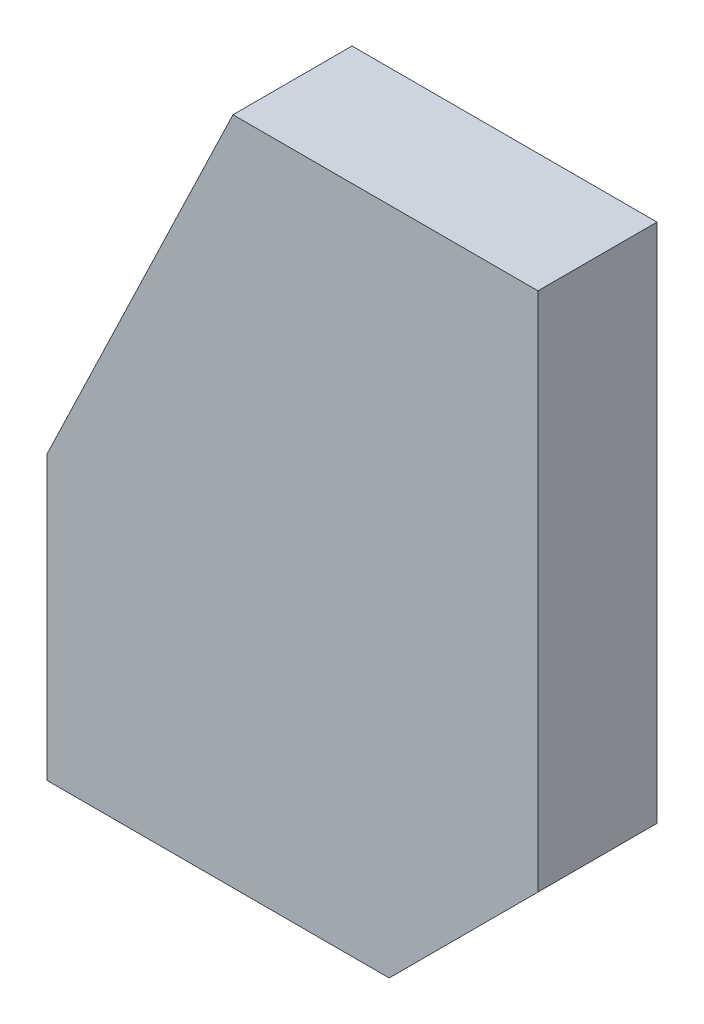
from build123d import *

# Parameters (mm, degrees)
EXTRUDE_1_DEPTH = 8
CHAMFER_1_SIZE  = 20


with BuildPart() as part:
    # 草图2 → 凸台-拉伸1 (new, symmetric)
    with BuildSketch(Plane.XY):
        Polygon((25, 90), (66, 90), (66, 0), (0, 0), (0, 38), align=None)
    extrude(amount=EXTRUDE_1_DEPTH, both=True)

    # 倒角1
    chamfer_1_edges = [part.edges().sort_by_distance(p)[0] for p in [
        (66, 0, 0),
    ]]
    chamfer(chamfer_1_edges, length=CHAMFER_1_SIZE)


solid = part.part
